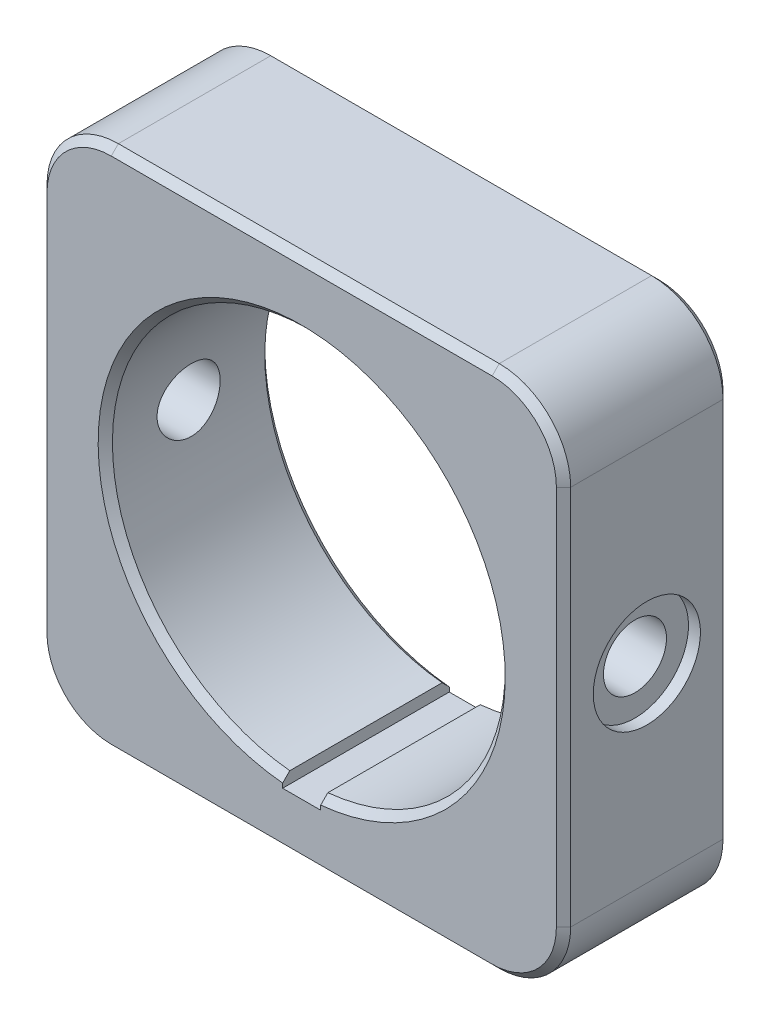
SolidWorks part; units mm, degrees
ref_plane "Front Plane" through (0, 0, 0) normal (0, 0, 1) x (1, 0, 0)
ref_plane "Top Plane" through (0, 0, 0) normal (0, 1, 0) x (1, 0, 0)
ref_plane "Right Plane" through (0, 0, 0) normal (1, 0, 0) x (0, 0, -1)
sketch "Sketch1" plane through (0, 0, 0) normal (0, 0, 1) x (1, 0, 0)
  line L1 (110, -110) -> (-110, -110)
  line L2 (110, -110) -> (110, 110)
  line L3 (110, 110) -> (-110, 110)
  line L4 (-110, -110) -> (-110, 110)
  line L5 (110, -110) -> (-110, 110) construction
  line L6 (110, 110) -> (-110, -110) construction
  point P0 (0, 0)
  dimension "D1" = 220
  dimension "D2" = 220
extrude "Boss-Extrude1" add sketch "Sketch1" along normal blind 70
sketch "Sketch2" plane through (0, 0, 70) normal (0, 0, 1) x (1, 0, 0)
  circle A0 centre (0, 0) radius 82.5
  dimension "D1" = 165
extrude "Cut-Extrude1" cut sketch "Sketch2" against normal through all
hole_wizard "M30 Tapped Hole1" positions "Sketch4" profile "Sketch5" tap size "M30" standard "GB" end condition through all
sketch "Sketch4" plane through (110, 0, 0) normal (1, 0, 0) x (0, 0, -1)
  line L0 (-35, 110) -> (-35, -110)
  line L1 (-70, 110) -> (0, 110) construction
  line L2 (-70, -110) -> (0, -110) construction
  point P0 (-35, 0)
sketch "Sketch5" plane through (110, 0, 35) normal (0, 1, 0) x (0, 0, -1)
  line L0 (0, 0) -> (0, 220)
  line L1 (0, 220) -> (13.25, 220)
  line L2 (13.25, 220) -> (13.25, 0)
  line L5 (13.25, 0) -> (0, 0)
  line L11 (0, -6.35) -> (0, 107.95) construction
  dimension "通孔螺纹孔钻头直径" = 26.5
  dimension "通孔螺纹孔钻头深度" = 220
cosmetic thread "Cosmetic thread 1" parameters "D2"=30
sketch "Sketch7" plane through (-110, 0, 0) normal (-1, 0, 0) x (0, 0, 1)
  circle A0 centre (35, 0) radius 22.5
  dimension "D1" = 45
extrude "Cut-Extrude3" cut sketch "Sketch7" against normal blind 5
mirror "Mirror1" about plane through (0, 0, 0) normal (1, 0, 0) of "Cut-Extrude3"
fillet "Fillet1" radius 30 4 edges at (110, 110, 35) (110, -110, 35) (-110, -110, 35) (-110, 110, 35)
chamfer "Chamfer1" distance 3 angle 45 18 edges at (-101.2132, 101.2132, 0) (-110, 0, 0) (-101.2132, -101.2132, 0) (0, -110, 0) (101.2132, -101.2132, 0) (110, 0, 0) (101.2132, 101.2132, 0) (0, 110, 0) (82.5, 0, 0) (101.2132, -101.2132, 70) (0, -110, 70) (-101.2132, -101.2132, 70) (-110, 0, 70) (-101.2132, 101.2132, 70) (0, 110, 70) (101.2132, 101.2132, 70) (110, 0, 70) (82.5, 0, 70)
sketch "Sketch8" plane through (0, 0, 0) normal (0, 0, -1) x (-1, 0, 0)
  line L0 (0, 0) -> (0, -57.1258) construction
  line L1 (8, 0) -> (-8, 0)
  line L2 (8, 0) -> (8, -87)
  line L3 (8, -87) -> (-8, -87)
  line L4 (-8, 0) -> (-8, -87)
  dimension "D1" = 16
  dimension "D2" = 87
extrude "Cut-Extrude4" cut sketch "Sketch8" against normal through all
